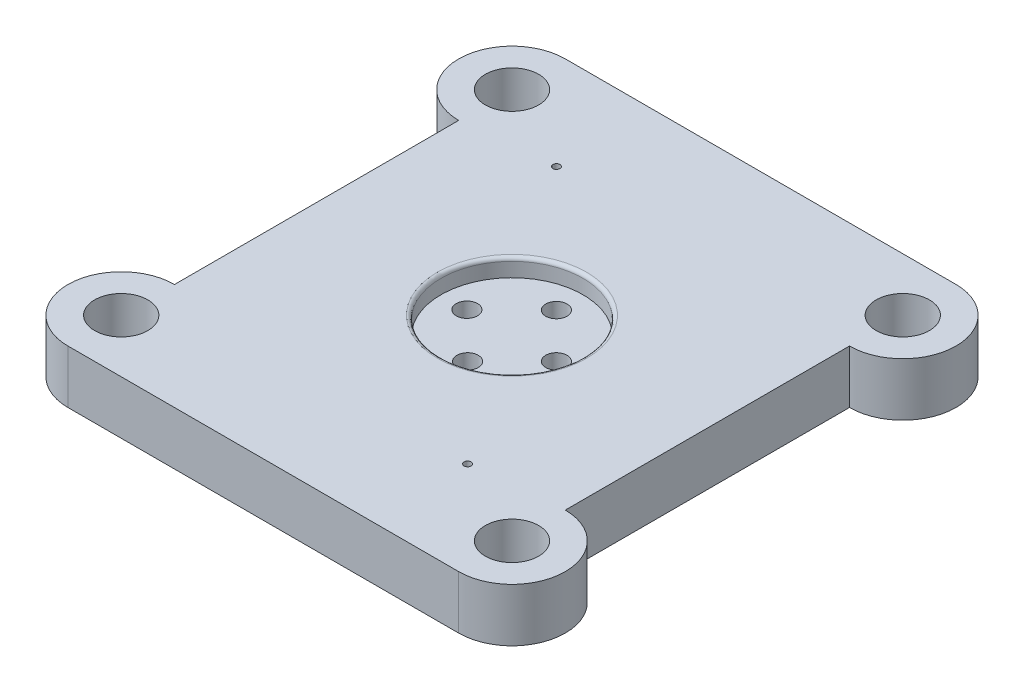
SolidWorks part; units mm, degrees
ref_plane "Front Plane" through (0, 0, 0) normal (0, 0, 1) x (1, 0, 0)
ref_plane "Top Plane" through (0, 0, 0) normal (0, 1, 0) x (1, 0, 0)
ref_plane "Right Plane" through (0, 0, 0) normal (1, 0, 0) x (0, 0, -1)
sketch "Sketch1" plane through (0, 0, 0) normal (0, 1, 0) x (1, 0, 0)
  line L0 (-110, -140) -> (80, -140)
  line L1 (80, -140) -> (80, 140)
  line L2 (80, 140) -> (-110, 140)
  line L7 (-110, -80) -> (-110, 80)
  arc A0 (-110, 140) -> (-110, 80) centre (-110, 110) ccw
  arc A1 (-110, -80) -> (-110, -140) centre (-110, -110) ccw
  circle A2 centre (-110, 110) radius 15
  circle A3 centre (-110, -110) radius 15
  dimension "D1" = 60
  dimension "D2" = 60
extrude "Boss-Extrude1" add sketch "Sketch1" along normal blind 30
ref_plane "Plane1" through (0, 0, 0) normal (0, 0, 1) x (1, 0, 0)
hole_wizard "CBORE for M8 Pan Head Machine Screw1" positions "Sketch4" profile "Sketch3" counterbore size "M8" standard "ANSI Metric" end condition through all
sketch "Sketch4" plane through (0, 30, 0) normal (0, 1, 0) x (1, 0, 0)
  line L0 (80, -140) -> (80, 140) construction
  line L1 (80, 140) -> (-110, 140) construction
  line L2 (-110, -140) -> (80, -140) construction
  point P0 (60, 120)
  point P2 (-60, 120)
  point P4 (-60, -120)
  point P6 (60, -120)
  dimension "D1" = 20
  dimension "D2" = 20
  dimension "D3" = 120
  dimension "D4" = 20
  dimension "D5" = 240
  dimension "D6" = 120
  dimension "D7" = 20
  dimension "D8" = 20
sketch "Sketch3" plane through (60, 30, -120) normal (1, 0, 0) x (0, 0, 1)
  line L0 (0, 0) -> (0, 30)
  line L1 (0, 30) -> (4.5, 30)
  line L3 (4.5, 30) -> (4.5, 6)
  line L4 (4.5, 6) -> (9, 6)
  line L5 (9, 6) -> (9, 0)
  line L7 (9, 0) -> (0, 0)
  line L11 (0, -6.35) -> (0, 107.95) construction
  dimension "Thru Hole Dia." = 9
  dimension "Thru Hole Depth" = 30
  dimension "C'Bore Dia." = 18
  dimension "C'Bore Depth" = 6
mirror "Mirror1" about plane through (0, 0, 0) normal (1, 0, 0) of "Boss-Extrude1"
sketch "草图1" plane through (0, 30, 0) normal (0, 1, 0) x (1, 0, 0)
  line L0 (0, 144.2948) -> (0, -158.1621) construction
  line L1 (-60, 144.2948) -> (-60, -152.915) construction
  line L2 (-123.6813, 0) -> (133.8007, 0) construction
  circle A0 centre (-60, 85) radius 2
  circle A1 centre (60, -85) radius 2
  dimension "D3" = 4
  dimension "D5" = 4
  dimension "D1" = 60
  dimension "D2" = 85
  dimension "D4" = 85
  dimension "D6" = 60
extrude "Cut-Extrude1" cut sketch "草图1" against normal through all
sketch "草图3" plane through (0, 0, 0) normal (0, -1, 0) x (1, 0, 0)
  line L0 (0, 148.0427) -> (0, -158.9117) construction
  line L1 (-120.3433, 0) -> (138.7049, 0) construction
  circle A0 centre (-60, 120) radius 5
  circle A1 centre (60, 120) radius 5
  circle A2 centre (60, -120) radius 5
  circle A3 centre (-60, -120) radius 5
  dimension "D1" = 10
  dimension "D2" = 60
  dimension "D3" = 120
extrude "Cut-Extrude3" cut sketch "草图3" against normal blind 20
sketch "草图4" plane through (0, 30, 0) normal (0, 1, 0) x (1, 0, 0)
  line L0 (0, -183.0116) -> (0, 207.2687) construction
  line L1 (-62.2638, 0) -> (127.04, 0) construction
  circle A0 centre (0, 0) radius 40
  dimension "D2" = 80
  dimension "D1" = 0
extrude "Cut-Extrude4" cut sketch "草图4" against normal blind 10
fillet "Fillet1" radius 2 1 edges at (0, 30, 40)
sketch "Sketch5" plane through (0, 20, 0) normal (0, 1, 0) x (1, 0, 0)
  line L0 (0, 0) -> (78.3315, 0) construction
  line L1 (0, 107.5652) -> (0, 28.859) construction
  circle A0 centre (0, 25) radius 6
  circle A1 centre (-25.4, 0) radius 6
  circle A4 centre (25, 0) radius 6
  circle A5 centre (0, -25) radius 6
  circle A6 centre (-25, 0) radius 6
  circle A7 centre (-50.4, 25.4) radius 6 [skipped]
  circle A8 centre (-25, 50.4) radius 6 [skipped]
  point P17 (-25.2, 25.2)
  point P24 (0, 0)
  dimension "D1" = 4
  dimension "D2" = 25
  dimension "D3" = 4
extrude "Cut-Extrude7" cut sketch "Sketch5" against normal blind 15 contours A0 | A1 | A5 | A4
